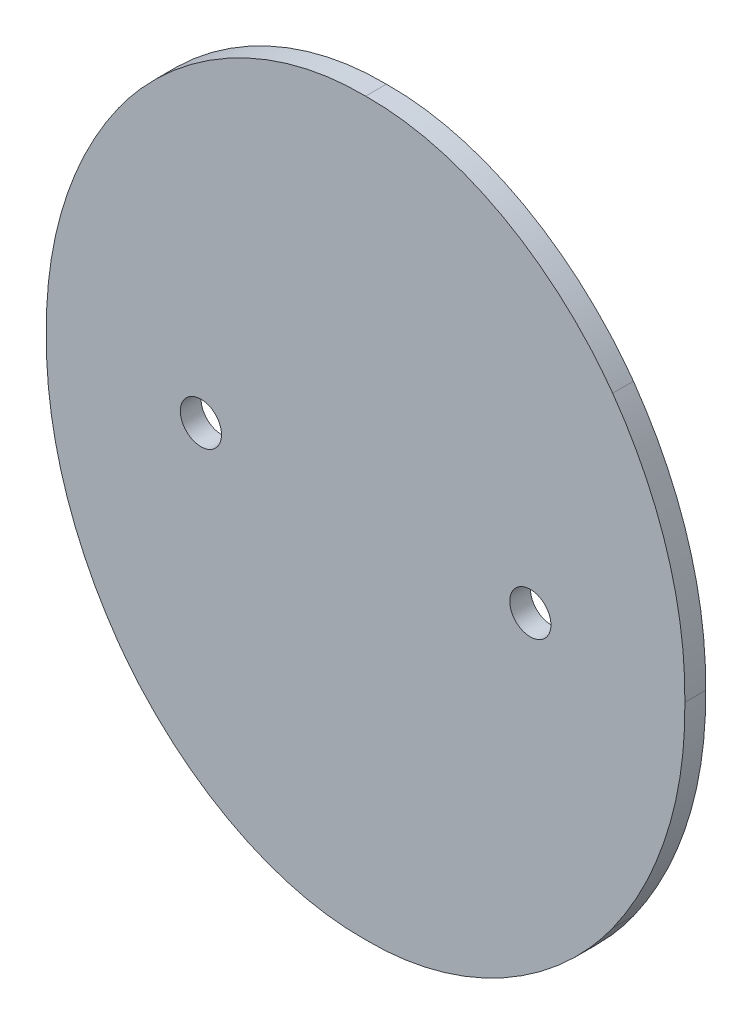
SolidWorks part; units mm, degrees
ref_plane "Front Plane" through (0, 0, 0) normal (0, 0, 1) x (1, 0, 0)
ref_plane "Top Plane" through (0, 0, 0) normal (0, 1, 0) x (1, 0, 0)
ref_plane "Right Plane" through (0, 0, 0) normal (1, 0, 0) x (0, 0, -1)
sketch "Sketch1" plane through (0, 0, 0) normal (0, 0, 1) x (1, 0, 0)
  line L0 (-68.7187, 0) -> (104.2297, 0) construction
  line L1 (0, -75.9168) -> (0, 76.6209) construction
  arc A0 (19.05, 17.8562) -> (24.6126, 0) centre (-5.4575, 0.427) cw
  arc A1 (-19.05, 17.8562) -> (-24.6126, 0) centre (5.4575, 0.427) ccw
  arc A2 (19.05, 17.8562) -> (24.6126, 0) centre (-5.4575, 0.427) cw
  arc A3 (-19.05, 17.8562) -> (-24.6126, 0) centre (5.4575, 0.427) ccw
  arc A4 (19.05, -17.8562) -> (24.6126, 0) centre (-5.4575, -0.427) ccw
  arc A5 (-19.05, -17.8562) -> (-24.6126, 0) centre (5.4575, -0.427) cw
  spline S0 degree 3 poles (0, 28.1686) (7.5778, 28.2851) (14.7191, 23.9101) (19.05, 17.8562) knots 0 0 0 0 1 1 1 1
  spline S1 degree 3 poles (0, 28.1686) (-7.5778, 28.2851) (-14.7191, 23.9101) (-19.05, 17.8562) knots 0 0 0 0 1 1 1 1
  spline S2 degree 3 poles (0, 28.1686) (7.5778, 28.2851) (14.7191, 23.9101) (19.05, 17.8562) knots 0 0 0 0 1 1 1 1
  spline S3 degree 3 poles (0, 28.1686) (-7.5778, 28.2851) (-14.7191, 23.9101) (-19.05, 17.8562) knots 0 0 0 0 1 1 1 1
  spline S4 degree 3 poles (0, -28.1686) (7.5778, -28.2851) (14.7191, -23.9101) (19.05, -17.8562) knots 0 0 0 0 1 1 1 1
  spline S5 degree 3 poles (0, -28.1686) (-7.5778, -28.2851) (-14.7191, -23.9101) (-19.05, -17.8562) knots 0 0 0 0 1 1 1 1
  dimension "D1" = 12.7
  dimension "D8" = 24.6126
  dimension "D2" = 6.35
  dimension "D3" = 27.2288
  dimension "D4" = 28.1686
  dimension "D5" = 24.1046
  dimension "D6" = 17.8562
  dimension "D7" = 19.05
extrude "Boss-Extrude1" add sketch "Sketch1" along normal blind 1.6002 contours S5 S4 A4 A0 S0 S1 A1 A5
sketch "Sketch2" plane through (0, 0, 1.6002) normal (0, 0, 1) x (1, 0, 0)
  line L0 (0, -16.3744) -> (0, 24.7609) construction
  line L1 (-33.1389, 0) -> (35.2021, 0) construction
  circle A0 centre (-12.7, 0) radius 1.5875
  circle A1 centre (12.7, 0) radius 1.5875
  dimension "D1" = 3.175
  dimension "D2" = 25.4
extrude "Cut-Extrude1" cut sketch "Sketch2" against normal blind 1.6002
